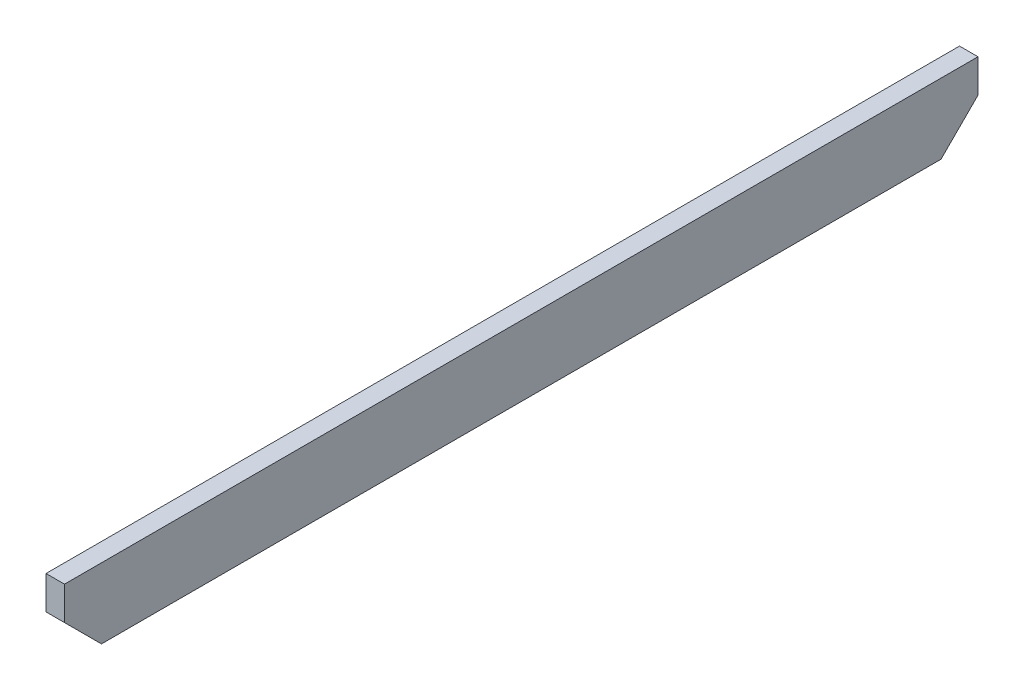
SolidWorks part; units mm, degrees
material "Q235A"
ref_plane "前视基准面" through (0, 0, 0) normal (0, 0, 1) x (1, 0, 0)
ref_plane "上视基准面" through (0, 0, 0) normal (0, 1, 0) x (1, 0, 0)
ref_plane "右视基准面" through (0, 0, 0) normal (1, 0, 0) x (0, 0, -1)
sketch3d "参数化"
  line L0 (-30.6165, 0, 0) -> (30.6165, 0, 0)
  line L1 (0, -14.0929, 0) -> (0, 14.0929, 0)
  line L2 (0, 0, 21.6949) -> (0, 0, -21.6949)
  point P4 (0, 0, 0)
  point P8 (0, 0, 0)
  point P11 (0, 0, 0)
sketch "草图1" plane through (0, 0, 0) normal (1, 0, 0) x (0, 0, -1)
  line L1 (-123.5, -9.5) -> (123.5, -9.5)
  line L2 (-123.5, -9.5) -> (-123.5, 9.5)
  line L3 (-123.5, 9.5) -> (123.5, 9.5)
  line L4 (123.5, -9.5) -> (123.5, 9.5)
  line L5 (-123.5, -9.5) -> (123.5, 9.5) construction
  line L6 (-123.5, 9.5) -> (123.5, -9.5) construction
  point P0 (0, 0)
  dimension "D1" = 247
  dimension "D2" = 19
extrude "凸台-拉伸1" add sketch "草图1" along normal mid plane 5
chamfer "倒角1" distance 10 angle 45 2 edges at (0, -9.5, -123.5) (0, -9.5, 123.5)
